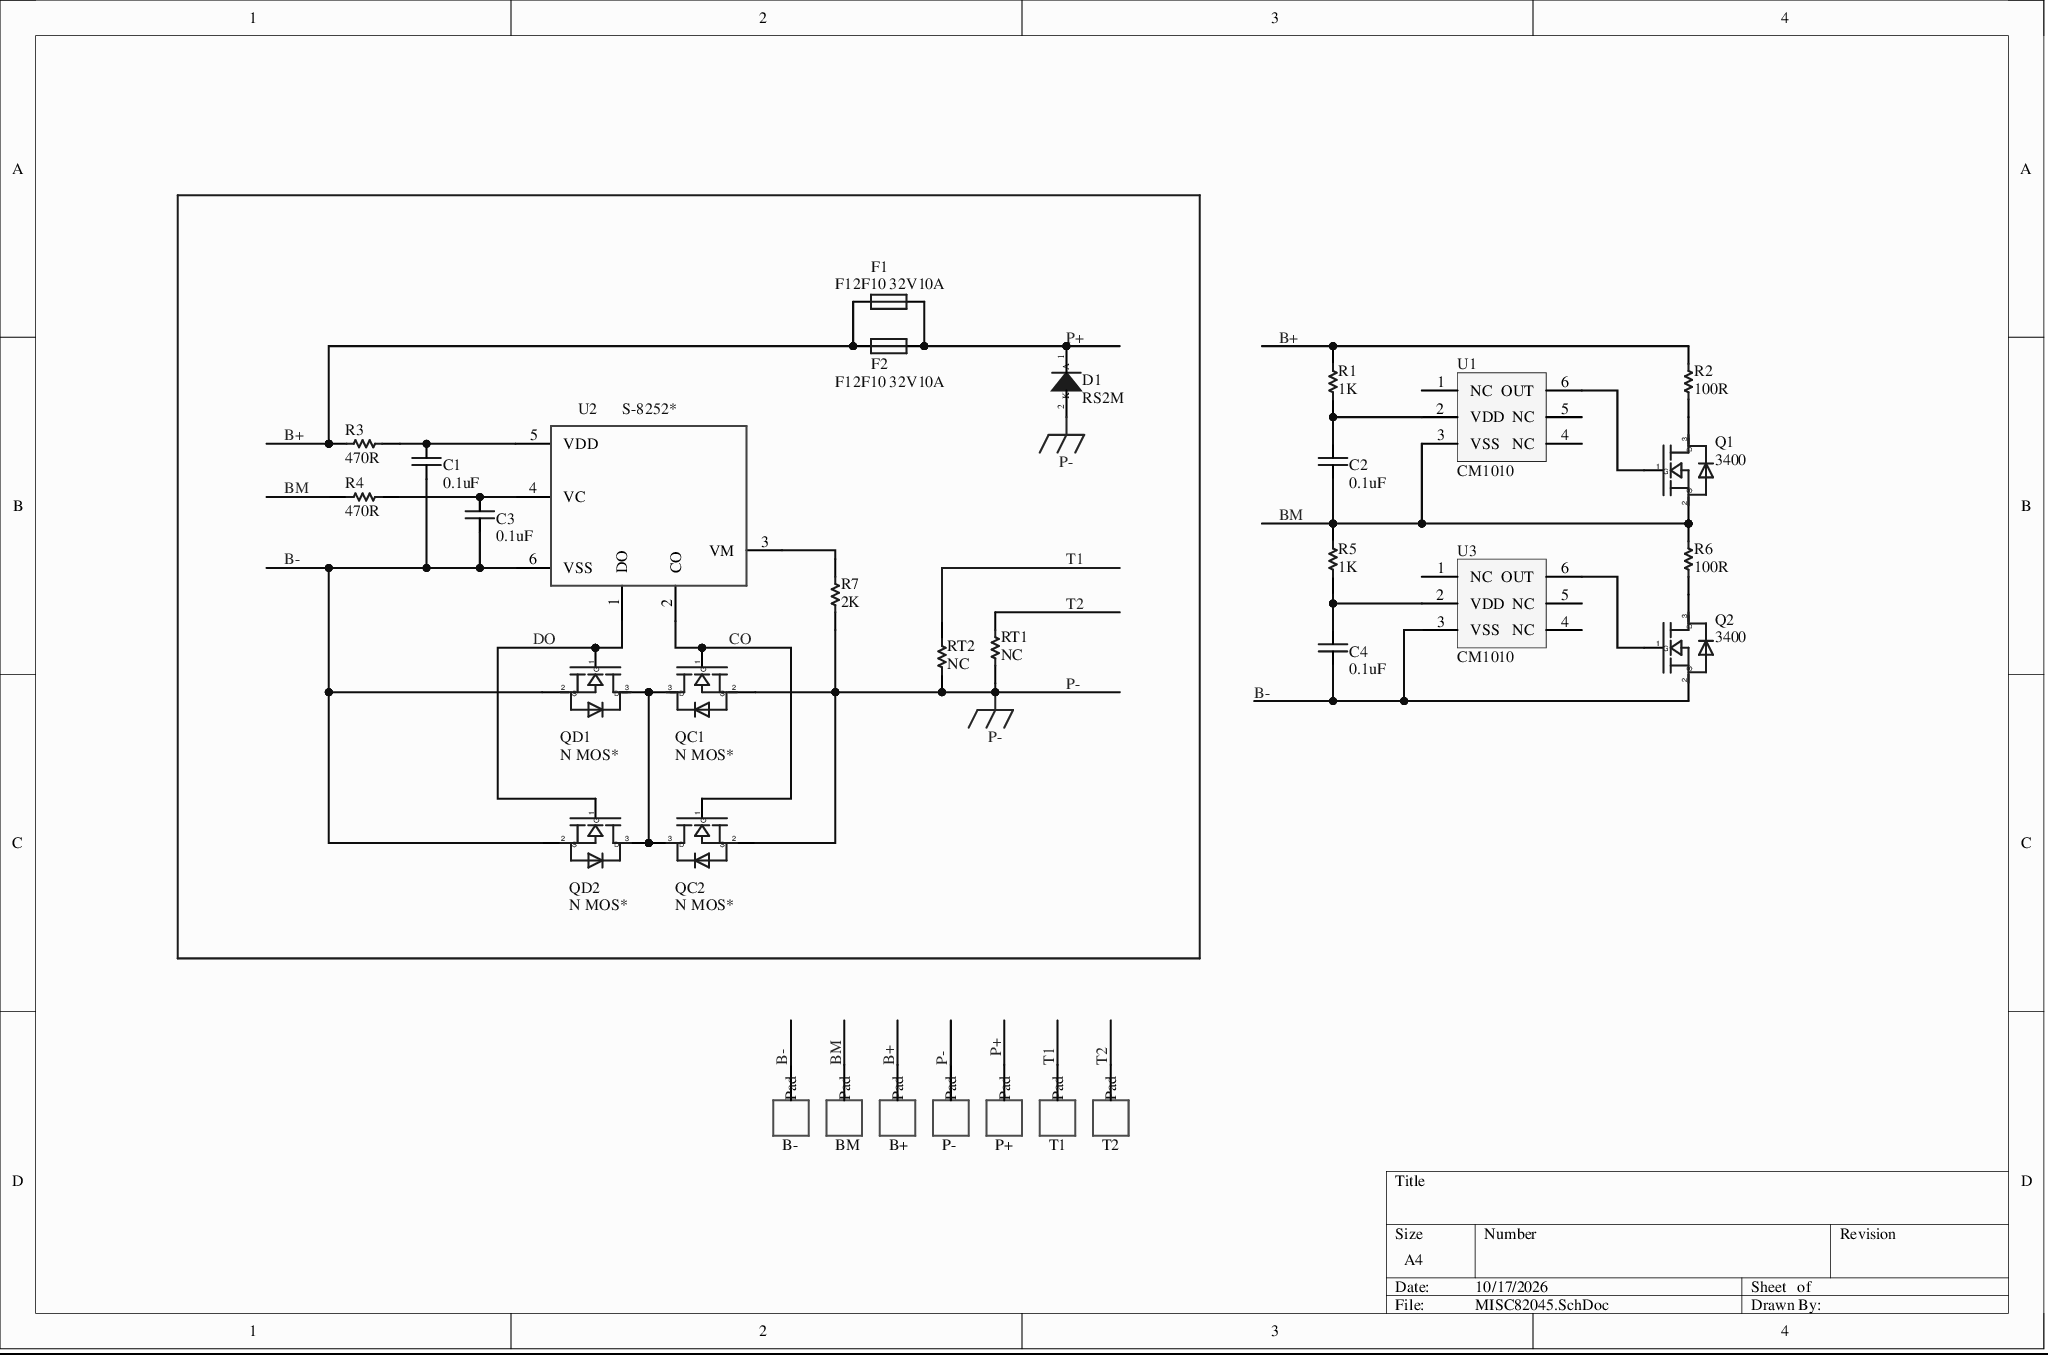
[diagram p0: MISC82045.SchDoc]
# Altium project MISC82045.PrjPcb
1 sheet, 32 parts. Net scope: global (net labels, ports and power ports of the same name join across sheets).
Board file: MISC82045.PcbDoc

## Sheet MISC82045.SchDoc
size A4; SheetNumber: 1; SheetTotal: 1

### Parts
B+  Pad  [Pad10X8mm]
B-  Pad  [Pad10X8mm]
BM  Pad  [Pad10X8mm]
C1  0.1uF  [C0603A]
C2  0.1uF  [C0603A]
C3  0.1uF  [C0603A]
C4  0.1uF  [C0603A]
D1  RS2M  [SMB A (1+2-)]
F1  F12F10 32V10A  [R1206A]
F2  F12F10 32V10A  [R1206A]
P+  Pad  [Pad10X8mm]
P-  Pad  [Pad10X8mm]
Q1  3400  [SOT23-3L]
Q2  3400  [SOT23-3L]
QC1  N MOS*  [TO-252]
QC2  N MOS*  [TO-252]
QD1  N MOS*  [TO-252]
QD2  N MOS*  [TO-252]
R1  1K  [R0603A]
R2  100R  [R1206A]
R3  470R  [R0603A]
R4  470R  [R0603A]
R5  1K  [R0603A]
R6  100R  [R1206A]
R7  2K  [R0603A]
RT1  NC  [R0603A]
RT2  NC  [R0603A]
T1  Pad  [Pad10X8mm]
T2  Pad  [Pad10X8mm]
U1  CM1010  [SOT23-6A]
U2  S-8252*  [SOT23-6A]
U3  CM1010  [SOT23-6A]

### Nets
P-: D1.2(K) P-.1 QC1.2(S) QC2.2(S) R7.1 RT1.1 RT2.1
B+: B+.1 F1.1 F2.1 R1.2 R2.2 R3.1
B-: B-.1 C1.1 C3.1 C4.1 Q2.2(S) QD1.2(S) QD2.2(S) U2.6(VSS) U3.3(VSS)
BM: BM.1 C2.1 Q1.2(S) R4.1 R5.2 R6.2 U1.3(VSS)
CO: QC1.1(G) QC2.1(G) U2.2(CO)
DO: QD1.1(G) QD2.1(G) U2.1(DO)
P+: D1.1(A) F1.2 F2.2 P+.1
T1: RT2.2 T1.1
T2: RT1.2 T2.1
NetC1_2: C1.2 R3.2 U2.5(VDD)
NetC2_2: C2.2 R1.1 U1.2(VDD)
NetC3_2: C3.2 R4.2 U2.4(VC)
NetC4_2: C4.2 R5.1 U3.2(VDD)
NetQ1_1: Q1.1(G) U1.6(OUT)
NetQ1_3: Q1.3(D) R2.1
NetQ2_1: Q2.1(G) U3.6(OUT)
NetQ2_3: Q2.3(D) R6.1
NetQC1_3: QC1.3(D) QC2.3(D) QD1.3(D) QD2.3(D)
NetR7_2: R7.2 U2.3(VM)

Not connected (* = marked no-connect by the designer): U1 1(NC)* 4(NC)* 5(NC)*; U3 1(NC)* 4(NC)* 5(NC)*

### Library data of the parts
B+ B- BM P+ P- T1 T2 = Pad: Connection pad (non-through-hole)
C1-C4 = CAP: SMD capacitor
D1 = RS2M: SMD diode
F1 F2 = FUSE
Q1 Q2 QC1 QC2 QD1 QD2 = N MOS*: SMD MOSFET
R1-R7 RT1 RT2 = RES: SMD resistor
U1 U3 = CM1010: Chuangxinwei, balancing IC
U2 = S-8252: 2S battery protection IC